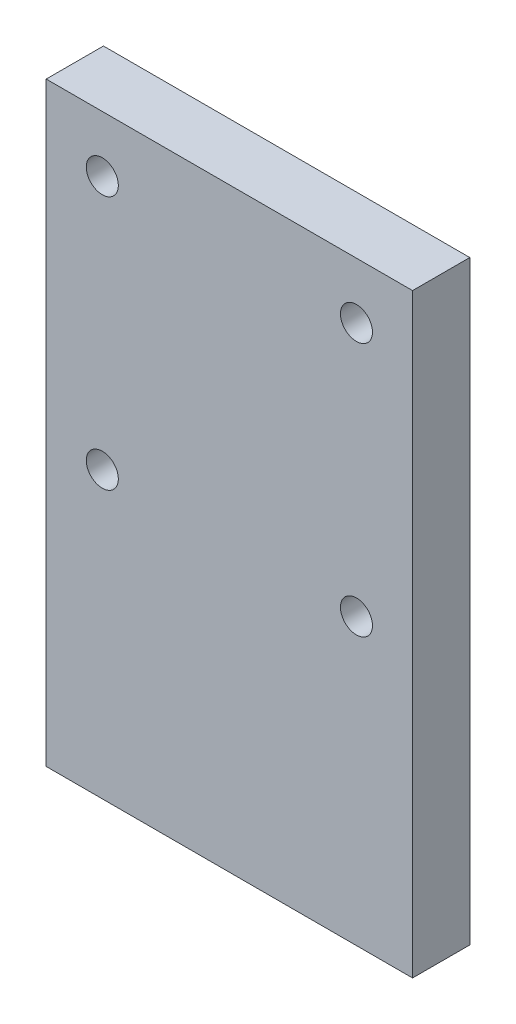
from build123d import *

# Parameters (mm, degrees)
SKETCH_1_W          = 160
SKETCH_1_H          = 260
EXTRUDE_1_DEPTH     = 25
HOLE_WIZARD_M16_1_D = 14


with BuildPart() as part:
    # 草图1 → 凸台-拉伸1 (new body)
    with BuildSketch(Plane.XY):
        Rectangle(SKETCH_1_W, SKETCH_1_H)
    extrude(amount=EXTRUDE_1_DEPTH)

    # M16 螺纹孔1 (through all)
    with Locations(Plane.XY.offset(25)):
        with Locations((-55.5, 105.5), (-55.5, -5.5), (55.5, -5.5), (55.5, 105.5)):
            Hole(HOLE_WIZARD_M16_1_D / 2)


solid = part.part
